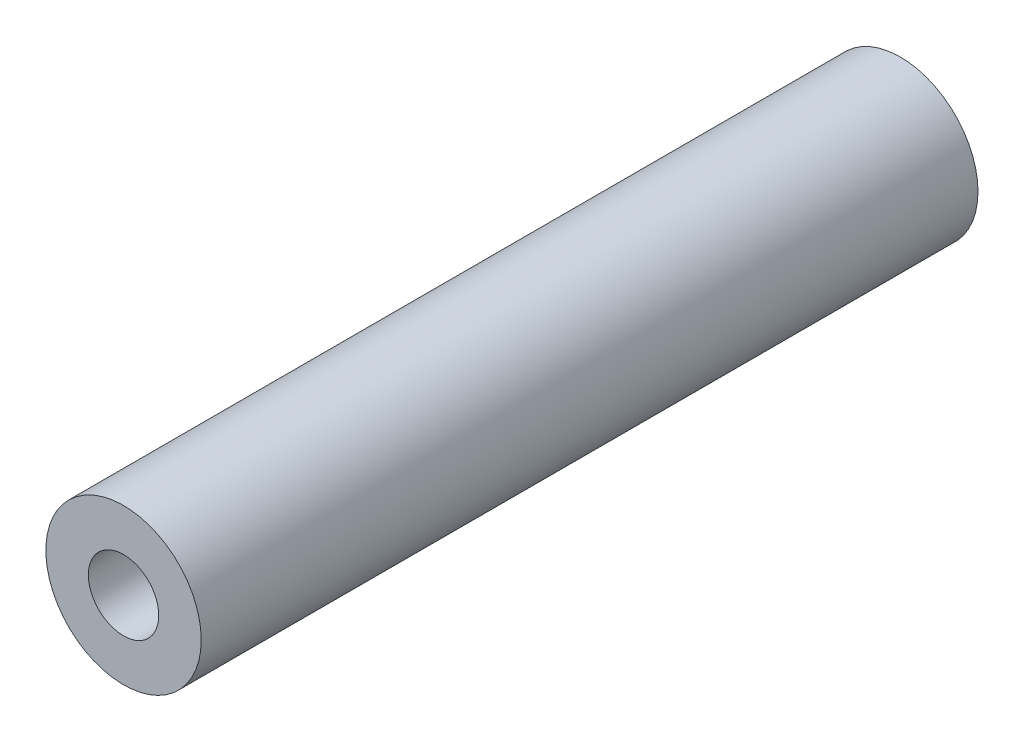
from build123d import *

# Parameters (mm, degrees)
SKETCH1_R             = 7.5
BOSS_EXTRUDE1_DEPTH   = 75
M8_TAPPED_HOLE1_D     = 6.8
M8_TAPPED_HOLE1_DEPTH = 19.75
M8_TAPPED_HOLE1_TIP   = 2.042926105
M8_TAPPED_HOLE2_D     = 6.8
M8_TAPPED_HOLE2_DEPTH = 19.75
M8_TAPPED_HOLE2_TIP   = 2.042926105


with BuildPart() as part:
    # Sketch1 → Boss-Extrude1 (new body)
    with BuildSketch(Plane.XY):
        Circle(SKETCH1_R)
    extrude(amount=BOSS_EXTRUDE1_DEPTH)

    # M8 Tapped Hole1
    with Locations(Plane.XY.offset(75)):
        with Locations((0, 0)):
            Hole(M8_TAPPED_HOLE1_D / 2, depth=M8_TAPPED_HOLE1_DEPTH)
            with Locations((0, 0, -(M8_TAPPED_HOLE1_DEPTH + M8_TAPPED_HOLE1_TIP / 2))):  # 118° drill point
                Cone(0, M8_TAPPED_HOLE1_D / 2, M8_TAPPED_HOLE1_TIP, mode=Mode.SUBTRACT)

    # M8 Tapped Hole2
    with Locations(Plane(origin=(0, 0, 0), x_dir=(-1, 0, 0), z_dir=(0, 0, -1))):
        with Locations((0, 0)):
            Hole(M8_TAPPED_HOLE2_D / 2, depth=M8_TAPPED_HOLE2_DEPTH)
            with Locations((0, 0, -(M8_TAPPED_HOLE2_DEPTH + M8_TAPPED_HOLE2_TIP / 2))):  # 118° drill point
                Cone(0, M8_TAPPED_HOLE2_D / 2, M8_TAPPED_HOLE2_TIP, mode=Mode.SUBTRACT)


solid = part.part
